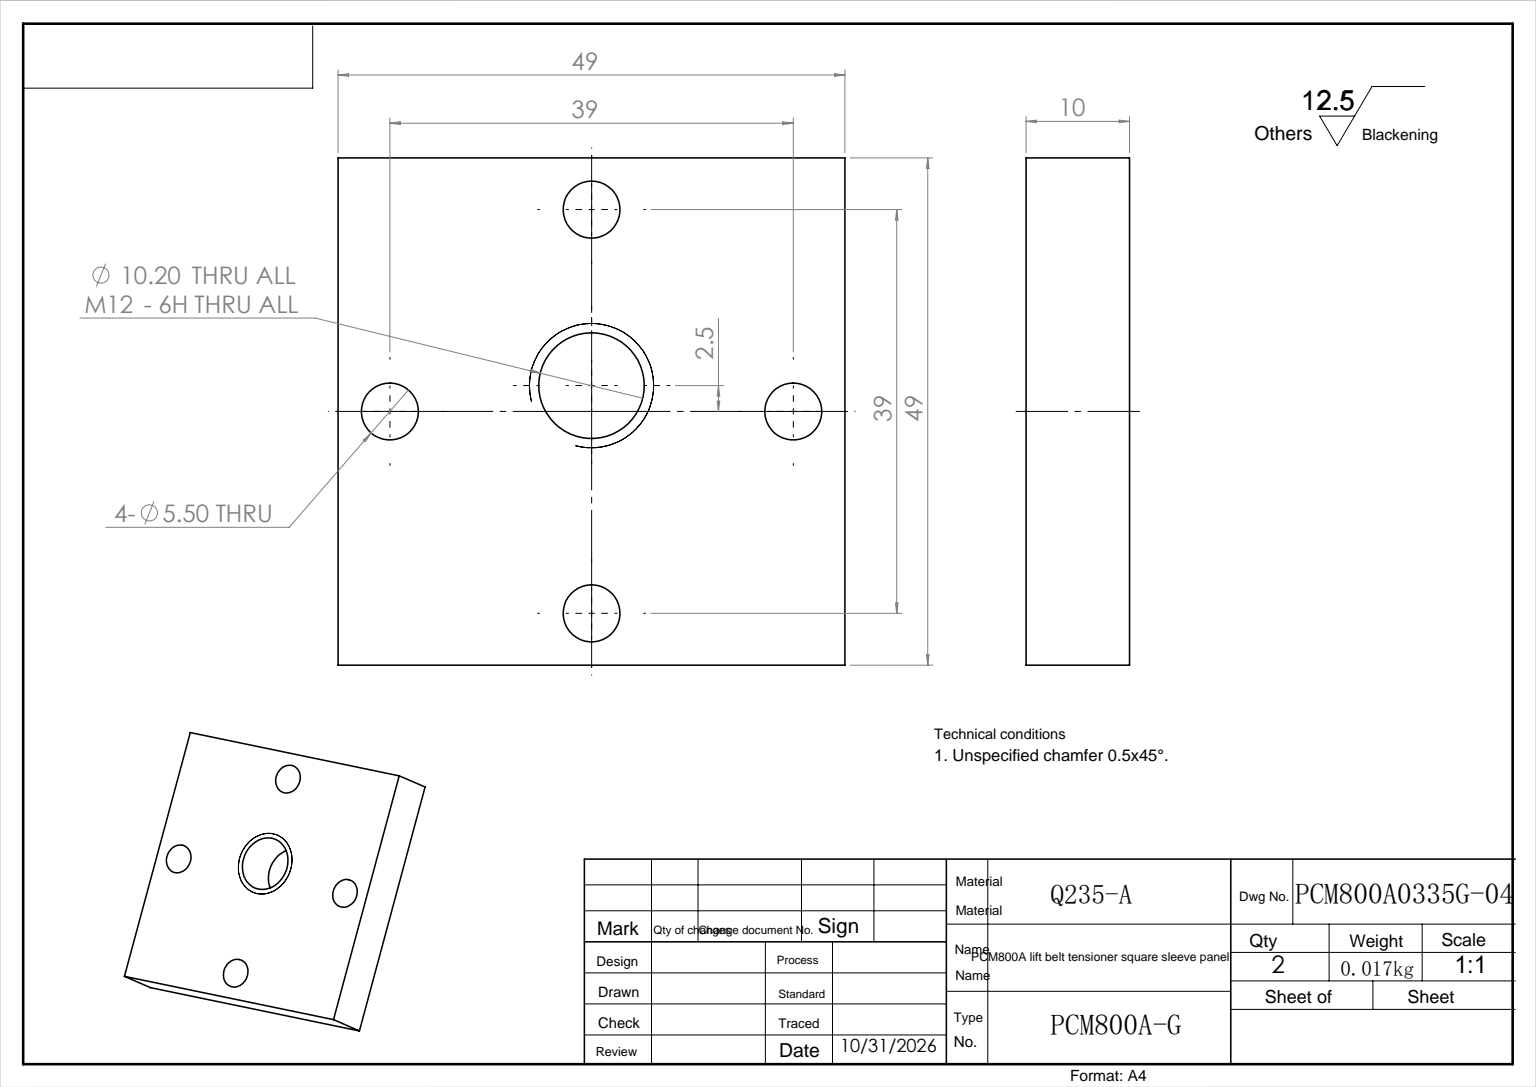
SolidWorks part; units mm, degrees
ref_plane "前视" through (0, 0, 0) normal (0, 0, 1) x (1, 0, 0)
ref_plane "上视" through (0, 0, 0) normal (0, 1, 0) x (1, 0, 0)
ref_plane "右视" through (0, 0, 0) normal (1, 0, 0) x (0, 0, -1)
sketch "草图1" plane through (0, 0, 0) normal (0, 1, 0) x (1, 0, 0)
  line L1 (0, 0) -> (49, 0)
  line L2 (0, 0) -> (0, 49)
  line L3 (0, 49) -> (49, 49)
  line L4 (49, 0) -> (49, 49)
  dimension "D1" = 49
  dimension "D2" = 49
extrude "拉伸1" add sketch "草图1" along normal blind 10
sketch "草图2" plane through (0, 10, 0) normal (0, 1, 0) x (-1, 0, 0)
  line L0 (-44, -44) -> (-44, -5) construction
  line L1 (-44, -5) -> (-5, -5) construction
  line L2 (-5, -5) -> (-5, -44) construction
  line L3 (-5, -44) -> (-44, -44) construction
  line L4 (-49, -49) -> (0, -49) construction
  line L5 (-49, 0) -> (-49, -49) construction
  line L6 (0, 0) -> (-49, 0) construction
  line L7 (0, -49) -> (0, 0) construction
  circle A0 centre (-24.5, -5) radius 2.75
  circle A1 centre (-44, -24.5) radius 2.75
  circle A2 centre (-24.5, -44) radius 2.75
  circle A3 centre (-5, -24.5) radius 2.75
  dimension "D5" = 5.5
  dimension "D6" = 5.5
  dimension "D7" = 5.5
  dimension "D8" = 5.5
  dimension "D1" = 5
  dimension "D2" = 5
  dimension "D3" = 5
  dimension "D4" = 5
extrude "切除-拉伸1" cut sketch "草图2" against normal through all
sketch "草图3" plane through (0, 10, 0) normal (0, 1, 0) x (-1, 0, 0)
  line L2 (0, -49) -> (0, 0) construction
  line L3 (-22.5, -49) -> (-22.5, 0) construction
  line L4 (-49, -49) -> (0, -49) construction
  line L5 (0, 0) -> (-49, 0) construction
  line L7 (-49, -27) -> (-22.5, -27) construction
  line L8 (-49, 0) -> (-49, -49) construction
  dimension "D1" = 22.5
  dimension "D2" = 27
hole_wizard "M12 螺纹孔1" positions "3D草图2" profile "草图5" tap size "M12" standard "GB" end condition through all
sketch3d "3D草图2"
  line L0 (49, 10, -24.5) -> (-5.5897, 10, -24.5) construction
  line L1 (49, 10, 0) -> (49, 10, -49) construction
  line L3 (24.5, 10, 0) -> (24.5, 10, -52.3593) construction
  line L4 (0, 10, 0) -> (49, 10, 0) construction
  point P16 (24.5, 10, -22)
  point P19 (24.5, 10, -22)
  dimension "D1" = 2.5
sketch "草图5" plane through (24.5, 10, -22) normal (1, 0, 0) x (0, 0, 1)
  line L0 (0, 0) -> (0, 10)
  line L1 (0, 10) -> (5.1, 10)
  line L2 (5.1, 10) -> (5.1, 0)
  line L5 (5.1, 0) -> (0, 0)
  line L11 (0, -6.35) -> (0, 107.95) construction
  dimension "通孔螺纹孔钻头直径" = 10.2
  dimension "通孔螺纹孔钻头深度" = 10
cosmetic thread "孔螺蚊线1" parameters "D2"=12
cosmetic thread "孔螺蚊线2" parameters "D2"=12
